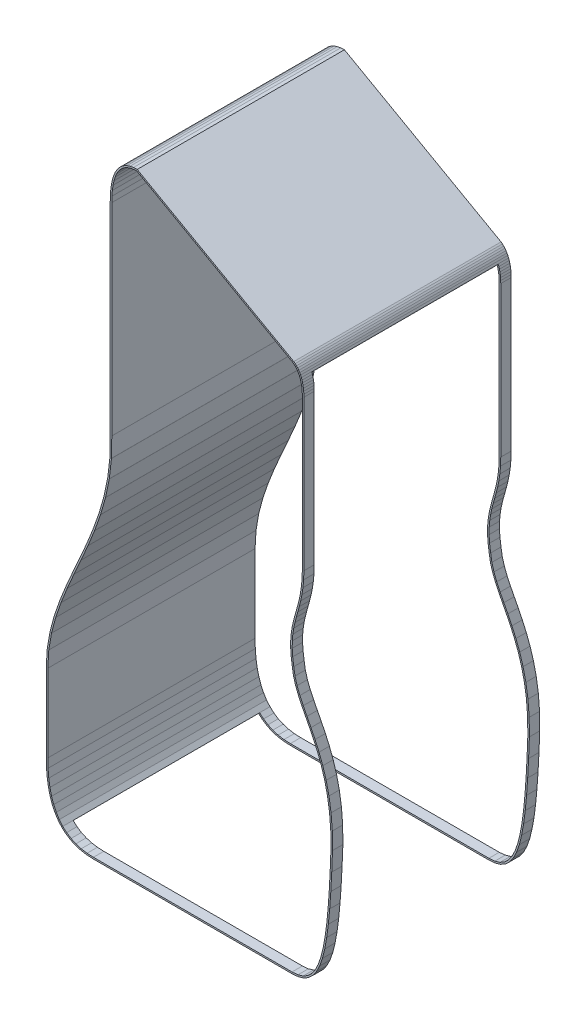
SolidWorks part; units mm, degrees
ref_plane "前视基准面" through (0, 0, 0) normal (0, 0, 1) x (1, 0, 0)
ref_plane "上视基准面" through (0, 0, 0) normal (0, 1, 0) x (1, 0, 0)
ref_plane "右视基准面" through (0, 0, 0) normal (1, 0, 0) x (0, 0, -1)
other "Configuration Table"
sketch "草图1" plane through (0, 0, 0) normal (0, 0, 1) x (1, 0, 0)
  line L0 (103, 235) -> (-24.8333, 235)
  line L1 (-24.8333, 235) -> (-152.6667, 235)
  line L2 (-152.6667, 235) -> (-280.5, 235)
  line L3 (-280.5, 235) -> (-293.0357, 235.6378)
  line L4 (-293.0357, 235.6378) -> (-304.6429, 237.551)
  line L5 (-304.6429, 237.551) -> (-315.3214, 240.7398)
  line L6 (-315.3214, 240.7398) -> (-325.0714, 245.2041)
  line L7 (-325.0714, 245.2041) -> (-333.8929, 250.9439)
  line L8 (-333.8929, 250.9439) -> (-341.7857, 257.9592)
  line L9 (-341.7857, 257.9592) -> (-348.75, 266.25)
  line L10 (-348.75, 266.25) -> (-354.7857, 275.8163)
  line L11 (-354.7857, 275.8163) -> (-359.8929, 286.6582)
  line L12 (-359.8929, 286.6582) -> (-364.0714, 298.7755)
  line L13 (-364.0714, 298.7755) -> (-367.3214, 312.1684)
  line L14 (-367.3214, 312.1684) -> (-369.6429, 326.8367)
  line L15 (-369.6429, 326.8367) -> (-371.0357, 342.7806)
  line L16 (-371.0357, 342.7806) -> (-371.5, 360)
  line L17 (-371.5, 360) -> (-371.5, 410)
  line L18 (-371.5, 410) -> (-371.5, 460)
  line L19 (-371.5, 460) -> (-371.5, 510)
  line L20 (-371.5, 510) -> (-369.6073, 541.7165)
  line L21 (-369.6073, 541.7165) -> (-364.3178, 572.7114)
  line L22 (-364.3178, 572.7114) -> (-356.2141, 603.1815)
  line L23 (-356.2141, 603.1815) -> (-345.879, 633.3236)
  line L24 (-345.879, 633.3236) -> (-333.8952, 663.3345)
  line L25 (-333.8952, 663.3345) -> (-320.8455, 693.4111)
  line L26 (-320.8455, 693.4111) -> (-307.3125, 723.75)
  line L27 (-307.3125, 723.75) -> (-293.879, 754.5481)
  line L28 (-293.879, 754.5481) -> (-281.1277, 786.0022)
  line L29 (-281.1277, 786.0022) -> (-269.6414, 818.309)
  line L30 (-269.6414, 818.309) -> (-260.0027, 851.6655)
  line L31 (-260.0027, 851.6655) -> (-252.7945, 886.2682)
  line L32 (-252.7945, 886.2682) -> (-248.5993, 922.3141)
  line L33 (-248.5993, 922.3141) -> (-248, 960)
  line L34 (-248, 960) -> (-248, 1090)
  line L35 (-248, 1090) -> (-248, 1220)
  line L36 (-248, 1220) -> (-248, 1350)
  line L37 (-248, 1350) -> (-247.7347, 1361.0204)
  line L38 (-247.7347, 1361.0204) -> (-246.9388, 1371.2245)
  line L39 (-246.9388, 1371.2245) -> (-245.6122, 1380.6122)
  line L40 (-245.6122, 1380.6122) -> (-243.7551, 1389.1837)
  line L41 (-243.7551, 1389.1837) -> (-241.3673, 1396.9388)
  line L42 (-241.3673, 1396.9388) -> (-238.449, 1403.8776)
  line L43 (-238.449, 1403.8776) -> (-235, 1410)
  line L44 (-235, 1410) -> (-231.0204, 1415.3061)
  line L45 (-231.0204, 1415.3061) -> (-226.5102, 1419.7959)
  line L46 (-226.5102, 1419.7959) -> (-221.4694, 1423.4694)
  line L47 (-221.4694, 1423.4694) -> (-215.898, 1426.3265)
  line L48 (-215.898, 1426.3265) -> (-209.7959, 1428.3673)
  line L49 (-209.7959, 1428.3673) -> (-203.1633, 1429.5918)
  line L50 (-203.1633, 1429.5918) -> (-196, 1430)
  line L51 (-196, 1430) -> (-95.25, 1373.3333)
  line L52 (-95.25, 1373.3333) -> (5.5, 1316.6667)
  line L53 (5.5, 1316.6667) -> (106.25, 1260)
  line L54 (106.25, 1260) -> (108.9362, 1257.8878)
  line L55 (108.9362, 1257.8878) -> (111.4235, 1255.551)
  line L56 (111.4235, 1255.551) -> (113.7117, 1252.9898)
  line L57 (113.7117, 1252.9898) -> (115.801, 1250.2041)
  line L58 (115.801, 1250.2041) -> (117.6913, 1247.1939)
  line L59 (117.6913, 1247.1939) -> (119.3827, 1243.9592)
  line L60 (119.3827, 1243.9592) -> (120.875, 1240.5)
  line L61 (120.875, 1240.5) -> (122.1684, 1236.8163)
  line L62 (122.1684, 1236.8163) -> (123.2628, 1232.9082)
  line L63 (123.2628, 1232.9082) -> (124.1582, 1228.7755)
  line L64 (124.1582, 1228.7755) -> (124.8546, 1224.4184)
  line L65 (124.8546, 1224.4184) -> (125.352, 1219.8367)
  line L66 (125.352, 1219.8367) -> (125.6505, 1215.0306)
  line L67 (125.6505, 1215.0306) -> (125.75, 1210)
  line L68 (125.75, 1210) -> (125.75, 1113.3333)
  line L69 (125.75, 1113.3333) -> (125.75, 1016.6667)
  line L70 (125.75, 1016.6667) -> (125.75, 920)
  line L71 (125.75, 920) -> (125.281, 904.7303)
  line L72 (125.281, 904.7303) -> (123.9876, 890.9038)
  line L73 (123.9876, 890.9038) -> (122.0405, 878.2799)
  line L74 (122.0405, 878.2799) -> (119.6101, 866.6181)
  line L75 (119.6101, 866.6181) -> (116.867, 855.6778)
  line L76 (116.867, 855.6778) -> (113.9818, 845.2187)
  line L77 (113.9818, 845.2187) -> (111.125, 835)
  line L78 (111.125, 835) -> (108.4672, 824.7813)
  line L79 (108.4672, 824.7813) -> (106.1789, 814.3222)
  line L80 (106.1789, 814.3222) -> (104.4308, 803.3819)
  line L81 (104.4308, 803.3819) -> (103.3932, 791.7201)
  line L82 (103.3932, 791.7201) -> (103.2369, 779.0962)
  line L83 (103.2369, 779.0962) -> (104.1323, 765.2697)
  line L84 (104.1323, 765.2697) -> (106.25, 750)
  line L85 (106.25, 750) -> (108.5868, 735.4045)
  line L86 (108.5868, 735.4045) -> (112.6079, 721.3994)
  line L87 (112.6079, 721.3994) -> (118.0076, 707.6567)
  line L88 (118.0076, 707.6567) -> (124.4803, 693.8484)
  line L89 (124.4803, 693.8484) -> (131.7206, 679.6465)
  line L90 (131.7206, 679.6465) -> (139.4227, 664.723)
  line L91 (139.4227, 664.723) -> (147.2812, 648.75)
  line L92 (147.2812, 648.75) -> (154.9905, 631.3994)
  line L93 (154.9905, 631.3994) -> (162.245, 612.3433)
  line L94 (162.245, 612.3433) -> (168.7391, 591.2536)
  line L95 (168.7391, 591.2536) -> (174.1672, 567.8025)
  line L96 (174.1672, 567.8025) -> (178.2238, 541.6618)
  line L97 (178.2238, 541.6618) -> (180.6032, 512.5036)
  line L98 (180.6032, 512.5036) -> (181, 480)
  line L99 (181, 480) -> (179.4934, 443.1706)
  line L100 (179.4934, 443.1706) -> (177.7026, 409.7522)
  line L101 (177.7026, 409.7522) -> (175.5423, 379.6356)
  line L102 (175.5423, 379.6356) -> (172.9271, 352.7114)
  line L103 (172.9271, 352.7114) -> (169.7719, 328.8703)
  line L104 (169.7719, 328.8703) -> (165.9913, 308.0029)
  line L105 (165.9913, 308.0029) -> (161.5, 290)
  line L106 (161.5, 290) -> (156.2128, 274.7522)
  line L107 (156.2128, 274.7522) -> (150.0445, 262.1501)
  line L108 (150.0445, 262.1501) -> (142.9096, 252.0845)
  line L109 (142.9096, 252.0845) -> (134.723, 244.4461)
  line L110 (134.723, 244.4461) -> (125.3994, 239.1254)
  line L111 (125.3994, 239.1254) -> (114.8535, 236.0131)
  line L112 (114.8535, 236.0131) -> (103, 235)
  line L113 (102.872, 238) -> (-280.4237, 238)
  line L114 (-280.4237, 238) -> (-292.7145, 238.6253)
  line L115 (-292.7145, 238.6253) -> (-303.967, 240.4801)
  line L116 (-303.967, 240.4801) -> (-314.2626, 243.5545)
  line L117 (-314.2626, 243.5545) -> (-323.621, 247.8395)
  line L118 (-323.621, 247.8395) -> (-332.0681, 253.3357)
  line L119 (-332.0681, 253.3357) -> (-339.6293, 260.0562)
  line L120 (-339.6293, 260.0562) -> (-346.3217, 268.0234)
  line L121 (-346.3217, 268.0234) -> (-352.1502, 277.2614)
  line L122 (-352.1502, 277.2614) -> (-357.1097, 287.7897)
  line L123 (-357.1097, 287.7897) -> (-361.1893, 299.6201)
  line L124 (-361.1893, 299.6201) -> (-364.3773, 312.7575)
  line L125 (-364.3773, 312.7575) -> (-366.6634, 327.2022)
  line L126 (-366.6634, 327.2022) -> (-368.0392, 342.9517)
  line L127 (-368.0392, 342.9517) -> (-368.5, 360.0404)
  line L128 (-368.5, 360.0404) -> (-368.5, 509.9106)
  line L129 (-368.5, 509.9106) -> (-366.6224, 541.3738)
  line L130 (-366.6224, 541.3738) -> (-361.3835, 572.0722)
  line L131 (-361.3835, 572.0722) -> (-353.342, 602.3084)
  line L132 (-353.342, 602.3084) -> (-343.0653, 632.2802)
  line L133 (-343.0653, 632.2802) -> (-331.1255, 662.181)
  line L134 (-331.1255, 662.181) -> (-318.0995, 692.2029)
  line L135 (-318.0995, 692.2029) -> (-304.5727, 722.5279)
  line L136 (-304.5727, 722.5279) -> (-304.5627, 722.5506)
  line L137 (-304.5627, 722.5506) -> (-291.1292, 753.3487)
  line L138 (-291.1292, 753.3487) -> (-291.0988, 753.421)
  line L139 (-291.0988, 753.421) -> (-278.3475, 784.8751)
  line L140 (-278.3475, 784.8751) -> (-278.3011, 784.9972)
  line L141 (-278.3011, 784.9972) -> (-266.8147, 817.3041)
  line L142 (-266.8147, 817.3041) -> (-266.7593, 817.4762)
  line L143 (-266.7593, 817.4762) -> (-257.1206, 850.8326)
  line L144 (-257.1206, 850.8326) -> (-257.0658, 851.0536)
  line L145 (-257.0658, 851.0536) -> (-249.8575, 885.6564)
  line L146 (-249.8575, 885.6564) -> (-249.8146, 885.9214)
  line L147 (-249.8146, 885.9214) -> (-245.6194, 921.9673)
  line L148 (-245.6194, 921.9673) -> (-245.5997, 922.2664)
  line L149 (-245.5997, 922.2664) -> (-245.0004, 959.9523)
  line L150 (-245.0004, 959.9523) -> (-245, 960)
  line L151 (-245, 960) -> (-245, 1349.9639)
  line L152 (-245, 1349.9639) -> (-244.7375, 1360.8676)
  line L153 (-244.7375, 1360.8676) -> (-243.9552, 1370.8977)
  line L154 (-243.9552, 1370.8977) -> (-242.6571, 1380.084)
  line L155 (-242.6571, 1380.084) -> (-240.8502, 1388.4233)
  line L156 (-240.8502, 1388.4233) -> (-238.5441, 1395.9133)
  line L157 (-238.5441, 1395.9133) -> (-235.7505, 1402.5554)
  line L158 (-235.7505, 1402.5554) -> (-232.4824, 1408.3568)
  line L159 (-232.4824, 1408.3568) -> (-228.7504, 1413.3328)
  line L160 (-228.7504, 1413.3328) -> (-224.5571, 1417.5072)
  line L161 (-224.5571, 1417.5072) -> (-219.8919, 1420.9069)
  line L162 (-219.8919, 1420.9069) -> (-214.7311, 1423.5535)
  line L163 (-214.7311, 1423.5535) -> (-209.0441, 1425.4554)
  line L164 (-209.0441, 1425.4554) -> (-202.8042, 1426.6074)
  line L165 (-202.8042, 1426.6074) -> (-196.7057, 1426.9549)
  line L166 (-196.7057, 1426.9549) -> (-96.7207, 1370.7185)
  line L167 (-96.7207, 1370.7185) -> (104.5776, 1257.4987)
  line L168 (104.5776, 1257.4987) -> (106.9782, 1255.611)
  line L169 (106.9782, 1255.611) -> (109.2737, 1253.4544)
  line L170 (109.2737, 1253.4544) -> (111.3889, 1251.0869)
  line L171 (111.3889, 1251.0869) -> (113.3265, 1248.5035)
  line L172 (113.3265, 1248.5035) -> (115.0877, 1245.6988)
  line L173 (115.0877, 1245.6988) -> (116.6723, 1242.6682)
  line L174 (116.6723, 1242.6682) -> (118.079, 1239.4076)
  line L175 (118.079, 1239.4076) -> (119.3056, 1235.914)
  line L176 (119.3056, 1235.914) -> (120.3497, 1232.1854)
  line L177 (120.3497, 1232.1854) -> (121.2088, 1228.2207)
  line L178 (121.2088, 1228.2207) -> (121.8803, 1224.0195)
  line L179 (121.8803, 1224.0195) -> (122.3621, 1219.5817)
  line L180 (122.3621, 1219.5817) -> (122.6523, 1214.9079)
  line L181 (122.6523, 1214.9079) -> (122.75, 1209.9703)
  line L182 (122.75, 1209.9703) -> (122.75, 920.0461)
  line L183 (122.75, 920.0461) -> (122.2853, 904.9163)
  line L184 (122.2853, 904.9163) -> (121.009, 891.2725)
  line L185 (121.009, 891.2725) -> (119.0875, 878.8149)
  line L186 (119.0875, 878.8149) -> (116.6855, 867.2892)
  line L187 (116.6855, 867.2892) -> (113.9656, 856.4416)
  line L188 (113.9656, 856.4416) -> (111.0912, 846.0214)
  line L189 (111.0912, 846.0214) -> (108.2358, 835.8077)
  line L190 (108.2358, 835.8077) -> (108.2216, 835.7552)
  line L191 (108.2216, 835.7552) -> (105.5638, 825.5365)
  line L192 (105.5638, 825.5365) -> (105.5365, 825.4225)
  line L193 (105.5365, 825.4225) -> (103.2483, 814.9633)
  line L194 (103.2483, 814.9633) -> (103.2165, 814.7955)
  line L195 (103.2165, 814.7955) -> (101.4683, 803.8553)
  line L196 (101.4683, 803.8553) -> (101.4426, 803.6478)
  line L197 (101.4426, 803.6478) -> (100.405, 791.986)
  line L198 (100.405, 791.986) -> (100.3935, 791.7573)
  line L199 (100.3935, 791.7573) -> (100.2371, 779.1334)
  line L200 (100.2371, 779.1334) -> (100.2432, 778.9023)
  line L201 (100.2432, 778.9023) -> (101.1386, 765.0758)
  line L202 (101.1386, 765.0758) -> (101.1607, 764.8576)
  line L203 (101.1607, 764.8576) -> (103.2784, 749.5879)
  line L204 (103.2784, 749.5879) -> (103.2877, 749.5257)
  line L205 (103.2877, 749.5257) -> (105.6246, 734.9302)
  line L206 (105.6246, 734.9302) -> (105.7033, 734.5766)
  line L207 (105.7033, 734.5766) -> (109.7244, 720.5715)
  line L208 (109.7244, 720.5715) -> (109.8157, 720.3023)
  line L209 (109.8157, 720.3023) -> (115.2154, 706.5596)
  line L210 (115.2154, 706.5596) -> (115.2912, 706.3834)
  line L211 (115.2912, 706.3834) -> (121.764, 692.5751)
  line L212 (121.764, 692.5751) -> (121.8076, 692.4858)
  line L213 (121.8076, 692.4858) -> (129.0479, 678.2839)
  line L214 (129.0479, 678.2839) -> (129.0547, 678.2706)
  line L215 (129.0547, 678.2706) -> (136.7436, 663.3728)
  line L216 (136.7436, 663.3728) -> (144.5635, 647.4783)
  line L217 (144.5635, 647.4783) -> (152.2158, 630.2558)
  line L218 (152.2158, 630.2558) -> (159.4066, 611.3672)
  line L219 (159.4066, 611.3672) -> (165.8405, 590.473)
  line L220 (165.8405, 590.473) -> (171.2196, 567.2334)
  line L221 (171.2196, 567.2334) -> (175.2426, 541.3093)
  line L222 (175.2426, 541.3093) -> (177.6047, 512.3632)
  line L223 (177.6047, 512.3632) -> (177.9993, 480.043)
  line L224 (177.9993, 480.043) -> (176.4967, 443.3121)
  line L225 (176.4967, 443.3121) -> (174.7084, 409.9398)
  line L226 (174.7084, 409.9398) -> (172.5527, 379.8879)
  line L227 (172.5527, 379.8879) -> (169.9462, 353.0533)
  line L228 (169.9462, 353.0533) -> (166.8072, 329.3347)
  line L229 (166.8072, 329.3347) -> (163.0568, 308.6341)
  line L230 (163.0568, 308.6341) -> (158.6217, 290.8562)
  line L231 (158.6217, 290.8562) -> (153.4381, 275.9073)
  line L232 (153.4381, 275.9073) -> (147.4566, 263.687)
  line L233 (147.4566, 263.687) -> (140.6392, 254.0692)
  line L234 (140.6392, 254.0692) -> (132.9322, 246.8782)
  line L235 (132.9322, 246.8782) -> (124.2156, 241.9039)
  line L236 (124.2156, 241.9039) -> (114.2955, 238.9764)
  line L237 (114.2955, 238.9764) -> (102.872, 238)
  point P0 (0, 0)
  dimension "D1" = 0.4643
  dimension "D2" = 1.8571
  dimension "D3" = 1.8927
  dimension "D4" = 3
  dimension "D5" = 3.4608
  dimension "D6" = 4.1786
  dimension "D7" = 4.8366
  dimension "D8" = 4.8776
  dimension "D9" = 7.1227
  dimension "D10" = 7.1822
  dimension "D11" = 7.4286
  dimension "D12" = 10.1165
  dimension "D13" = 10.3107
  dimension "D14" = 11.6071
  dimension "D15" = 14.3903
  dimension "D16" = 15.2859
  dimension "D17" = 16.7143
  dimension "D18" = 18.158
  dimension "D19" = 19.3498
  dimension "D20" = 22.75
  dimension "D21" = 25.1783
  dimension "D22" = 25.621
  dimension "D23" = 28.4347
  dimension "D24" = 29.7143
  dimension "D25" = 31.8707
  dimension "D26" = 37.6048
  dimension "D27" = 37.6071
  dimension "D28" = 39.4319
  dimension "D29" = 40.3745
  dimension "D30" = 46.4286
  dimension "D31" = 47.879
  dimension "D32" = 50.6545
  dimension "D33" = 53.4005
  dimension "D34" = 56.1786
  dimension "D35" = 57.2374
  dimension "D36" = 64.1875
  dimension "D37" = 66.8571
  dimension "D38" = 66.9273
  dimension "D39" = 66.9373
  dimension "D40" = 67.533
  dimension "D41" = 77.621
  dimension "D42" = 78.4643
  dimension "D43" = 78.7855
  dimension "D44" = 80.3708
  dimension "D45" = 80.4012
  dimension "D46" = 90.3723
  dimension "D47" = 91
  dimension "D48" = 91.0763
  dimension "D49" = 93.1525
  dimension "D50" = 93.1989
  dimension "D51" = 101.8586
  dimension "D52" = 104.6853
  dimension "D53" = 104.7407
  dimension "D54" = 111.4973
  dimension "D55" = 114.3794
  dimension "D56" = 114.4342
  dimension "D57" = 118.7055
  dimension "D58" = 121.6425
  dimension "D59" = 121.6854
  dimension "D60" = 122.9007
  dimension "D61" = 123.5
  dimension "D62" = 123.7653
  dimension "D63" = 124.5612
  dimension "D64" = 125.8806
  dimension "D65" = 125.8878
  dimension "D66" = 125.9003
  dimension "D67" = 126.4996
  dimension "D68" = 126.5
  dimension "D69" = 126.7625
  dimension "D70" = 127.5448
  dimension "D71" = 127.7449
  dimension "D72" = 128.8429
  dimension "D73" = 130.1327
  dimension "D74" = 130.6498
  dimension "D75" = 132.9559
  dimension "D76" = 133.051
  dimension "D77" = 135.7495
  dimension "D78" = 136.5
  dimension "D79" = 139.0176
  dimension "D80" = 140.4796
  dimension "D81" = 142.7496
  dimension "D82" = 144.9898
  dimension "D83" = 146.9429
  dimension "D84" = 150.0306
  dimension "D85" = 151.6081
  dimension "D86" = 155.602
  dimension "D87" = 156.7689
  dimension "D88" = 161.7041
  dimension "D89" = 162.4559
  dimension "D90" = 168.3367
  dimension "D91" = 168.6958
  dimension "D92" = 174.7943
  dimension "D93" = 175.5
  dimension "D94" = 218.8333
  dimension "D95" = 274.7793
  dimension "D96" = 276.25
  dimension "D97" = 346.6667
  dimension "D98" = 371.5
  dimension "D99" = 377
  dimension "D100" = 471.7371
  dimension "D101" = 471.7432
  dimension "D102" = 471.8935
  dimension "D103" = 471.905
  dimension "D104" = 472.6386
  dimension "D105" = 472.6607
  dimension "D106" = 472.9426
  dimension "D107" = 472.9683
  dimension "D108" = 474.372
  dimension "D109" = 474.5
  dimension "D110" = 474.7165
  dimension "D111" = 474.7369
  dimension "D112" = 474.7483
  dimension "D113" = 474.7784
  dimension "D114" = 474.7877
  dimension "D115" = 474.8932
  dimension "D116" = 475.6323
  dimension "D117" = 475.9308
  dimension "D118" = 476.0776
  dimension "D119" = 477.0365
  dimension "D120" = 477.0638
  dimension "D121" = 477.1246
  dimension "D122" = 477.2033
  dimension "D123" = 477.6789
  dimension "D124" = 477.75
  dimension "D125" = 478.4782
  dimension "D126" = 479.7216
  dimension "D127" = 479.7358
  dimension "D128" = 479.9672
  dimension "D129" = 480.0868
  dimension "D130" = 480.4362
  dimension "D131" = 480.7737
  dimension "D132" = 481.2244
  dimension "D133" = 481.3157
  dimension "D134" = 482.5912
  dimension "D135" = 482.625
  dimension "D136" = 482.8889
  dimension "D137" = 482.9235
  dimension "D138" = 484.1079
  dimension "D139" = 484.8265
  dimension "D140" = 485.2117
  dimension "D141" = 485.4656
  dimension "D142" = 485.4818
  dimension "D143" = 485.7955
  dimension "D144" = 486.3535
  dimension "D145" = 486.5877
  dimension "D146" = 486.7154
  dimension "D147" = 486.7912
  dimension "D148" = 487.301
  dimension "D149" = 488.1723
  dimension "D150" = 488.1855
  dimension "D151" = 488.367
  dimension "D152" = 489.1913
  dimension "D153" = 489.5076
  dimension "D154" = 489.579
  dimension "D155" = 490.5875
  dimension "D156" = 490.8056
  dimension "D157" = 490.8827
  dimension "D158" = 491.1101
  dimension "D159" = 491.8497
  dimension "D160" = 492.375
  dimension "D161" = 492.509
  dimension "D162" = 492.7088
  dimension "D163" = 493.264
  dimension "D164" = 493.3076
  dimension "D165" = 493.3803
  dimension "D166" = 493.5405
  dimension "D167" = 493.6684
  dimension "D168" = 493.7853
  dimension "D169" = 493.8621
  dimension "D170" = 494.1523
  dimension "D171" = 494.25
  dimension "D172" = 494.7628
  dimension "D173" = 495.4876
  dimension "D174" = 495.6582
  dimension "D175" = 495.7156
  dimension "D176" = 495.9803
  dimension "D177" = 496.3546
  dimension "D178" = 496.781
  dimension "D179" = 496.852
  dimension "D180" = 496.8994
  dimension "D181" = 497.1505
  dimension "D182" = 497.25
  dimension "D183" = 500.5479
  dimension "D184" = 500.5547
  dimension "D185" = 503.2206
  dimension "D186" = 504.4322
  dimension "D187" = 506.223
  dimension "D188" = 508.2436
  dimension "D189" = 510.9227
  dimension "D190" = 512.1392
  dimension "D191" = 514.4096
  dimension "D192" = 516.0635
  dimension "D193" = 518.7812
  dimension "D194" = 518.9566
  dimension "D195" = 521.5445
  dimension "D196" = 523.7158
  dimension "D197" = 524.9381
  dimension "D198" = 526.4905
  dimension "D199" = 527.7128
  dimension "D200" = 530.1217
  dimension "D201" = 530.9066
  dimension "D202" = 533
  dimension "D203" = 533.745
  dimension "D204" = 534.5568
  dimension "D205" = 537.3405
  dimension "D206" = 537.4913
  dimension "D207" = 538.3072
  dimension "D208" = 540.2391
  dimension "D209" = 541.2719
  dimension "D210" = 541.4462
  dimension "D211" = 542.7196
  dimension "D212" = 544.0527
  dimension "D213" = 544.4271
  dimension "D214" = 545.6672
  dimension "D215" = 546.2084
  dimension "D216" = 546.7426
  dimension "D217" = 547.0423
  dimension "D218" = 547.9967
  dimension "D219" = 549.1047
  dimension "D220" = 549.2026
  dimension "D221" = 549.4993
  dimension "D222" = 549.7238
  dimension "D223" = 550.9934
  dimension "D224" = 552.1032
  dimension "D225" = 552.5
  dimension "D226" = 0.6378
  dimension "D227" = 1.0131
  dimension "D228" = 2.551
  dimension "D229" = 3
  dimension "D230" = 3.6253
  dimension "D231" = 3.9764
  dimension "D232" = 4.1254
  dimension "D233" = 5.4801
  dimension "D234" = 5.7398
  dimension "D235" = 6.9039
  dimension "D236" = 8.5545
  dimension "D237" = 9.4461
  dimension "D238" = 10.2041
  dimension "D239" = 11.8782
  dimension "D240" = 12.8395
  dimension "D241" = 15.9439
  dimension "D242" = 17.0845
  dimension "D243" = 18.3357
  dimension "D244" = 19.0692
  dimension "D245" = 22.9592
  dimension "D246" = 25.0562
  dimension "D247" = 27.1501
  dimension "D248" = 28.687
  dimension "D249" = 31.25
  dimension "D250" = 33.0234
  dimension "D251" = 39.7522
  dimension "D252" = 40.8163
  dimension "D253" = 40.9073
  dimension "D254" = 42.2614
  dimension "D255" = 51.6582
  dimension "D256" = 52.7897
  dimension "D257" = 55
  dimension "D258" = 55.8562
  dimension "D259" = 63.7755
  dimension "D260" = 64.6201
  dimension "D261" = 73.0029
  dimension "D262" = 73.6341
  dimension "D263" = 77.1684
  dimension "D264" = 77.7575
  dimension "D265" = 91.8367
  dimension "D266" = 92.2022
  dimension "D267" = 93.8703
  dimension "D268" = 94.3347
  dimension "D269" = 107.7806
  dimension "D270" = 107.9517
  dimension "D271" = 117.7114
  dimension "D272" = 118.0533
  dimension "D273" = 125
  dimension "D274" = 125.0404
  dimension "D275" = 144.6356
  dimension "D276" = 144.8879
  dimension "D277" = 174.7522
  dimension "D278" = 174.9398
  dimension "D279" = 175
  dimension "D280" = 208.1706
  dimension "D281" = 208.3121
  dimension "D282" = 225
  dimension "D283" = 245
  dimension "D284" = 245.043
  dimension "D285" = 274.9106
  dimension "D286" = 275
  dimension "D287" = 277.3632
  dimension "D288" = 277.5036
  dimension "D289" = 306.3093
  dimension "D290" = 306.3738
  dimension "D291" = 306.6618
  dimension "D292" = 306.7165
  dimension "D293" = 332.2334
  dimension "D294" = 332.8025
  dimension "D295" = 337.0722
  dimension "D296" = 337.7114
  dimension "D297" = 355.473
  dimension "D298" = 356.2536
  dimension "D299" = 367.3084
  dimension "D300" = 368.1815
  dimension "D301" = 376.3672
  dimension "D302" = 377.3433
  dimension "D303" = 395.2558
  dimension "D304" = 396.3994
  dimension "D305" = 397.2802
  dimension "D306" = 398.3236
  dimension "D307" = 412.4783
  dimension "D308" = 413.75
  dimension "D309" = 427.181
  dimension "D310" = 428.3345
  dimension "D311" = 428.3728
  dimension "D312" = 429.723
  dimension "D313" = 443.2706
  dimension "D314" = 443.2839
  dimension "D315" = 444.6465
  dimension "D316" = 457.2029
  dimension "D317" = 457.4858
  dimension "D318" = 457.5751
  dimension "D319" = 458.4111
  dimension "D320" = 458.8484
  dimension "D321" = 471.3834
  dimension "D322" = 471.5596
  dimension "D323" = 472.6567
  dimension "D324" = 485.3023
  dimension "D325" = 485.5715
  dimension "D326" = 486.3994
  dimension "D327" = 487.5279
  dimension "D328" = 487.5506
  dimension "D329" = 488.75
  dimension "D330" = 499.5766
  dimension "D331" = 499.9302
  dimension "D332" = 500.4045
  dimension "D333" = 514.5257
  dimension "D334" = 514.5879
  dimension "D335" = 515
  dimension "D336" = 518.3487
  dimension "D337" = 518.421
  dimension "D338" = 519.5481
  dimension "D339" = 529.8576
  dimension "D340" = 530.0758
  dimension "D341" = 530.2697
  dimension "D342" = 543.9023
  dimension "D343" = 544.0962
  dimension "D344" = 544.1334
  dimension "D345" = 549.8751
  dimension "D346" = 549.9972
  dimension "D347" = 551.0022
  dimension "D348" = 556.7201
  dimension "D349" = 556.7573
  dimension "D350" = 556.986
  dimension "D351" = 568.3819
  dimension "D352" = 568.6478
  dimension "D353" = 568.8553
  dimension "D354" = 579.3222
  dimension "D355" = 579.7955
  dimension "D356" = 579.9633
  dimension "D357" = 582.3041
  dimension "D358" = 582.4762
  dimension "D359" = 583.309
  dimension "D360" = 589.7813
  dimension "D361" = 590.4225
  dimension "D362" = 590.5365
  dimension "D363" = 600
  dimension "D364" = 600.7552
  dimension "D365" = 600.8077
  dimension "D366" = 610.2187
  dimension "D367" = 611.0214
  dimension "D368" = 615.8326
  dimension "D369" = 616.0536
  dimension "D370" = 616.6655
  dimension "D371" = 620.6778
  dimension "D372" = 621.4416
  dimension "D373" = 631.6181
  dimension "D374" = 632.2892
  dimension "D375" = 643.2799
  dimension "D376" = 643.8149
  dimension "D377" = 650.6564
  dimension "D378" = 650.9214
  dimension "D379" = 651.2682
  dimension "D380" = 655.9038
  dimension "D381" = 656.2725
  dimension "D382" = 669.7303
  dimension "D383" = 669.9163
  dimension "D384" = 685
  dimension "D385" = 685.0461
  dimension "D386" = 686.9673
  dimension "D387" = 687.2664
  dimension "D388" = 687.3141
  dimension "D389" = 724.9523
  dimension "D390" = 725
  dimension "D391" = 781.6667
  dimension "D392" = 855
  dimension "D393" = 878.3333
  dimension "D394" = 974.9703
  dimension "D395" = 975
  dimension "D396" = 979.9079
  dimension "D397" = 980.0306
  dimension "D398" = 984.5817
  dimension "D399" = 984.8367
  dimension "D400" = 985
  dimension "D401" = 989.0195
  dimension "D402" = 989.4184
  dimension "D403" = 993.2207
  dimension "D404" = 993.7755
  dimension "D405" = 997.1854
  dimension "D406" = 997.9082
  dimension "D407" = 1000.914
  dimension "D408" = 1001.8163
  dimension "D409" = 1004.4076
  dimension "D410" = 1005.5
  dimension "D411" = 1007.6682
  dimension "D412" = 1008.9592
  dimension "D413" = 1010.6988
  dimension "D414" = 1012.1939
  dimension "D415" = 1013.5035
  dimension "D416" = 1015.2041
  dimension "D417" = 1016.0869
  dimension "D418" = 1017.9898
  dimension "D419" = 1018.4544
  dimension "D420" = 1020.551
  dimension "D421" = 1020.611
  dimension "D422" = 1022.4987
  dimension "D423" = 1022.8878
  dimension "D424" = 1025
  dimension "D425" = 1081.6667
  dimension "D426" = 1114.9639
  dimension "D427" = 1115
  dimension "D428" = 1125.8676
  dimension "D429" = 1126.0204
  dimension "D430" = 1135.7185
  dimension "D431" = 1135.8977
  dimension "D432" = 1136.2245
  dimension "D433" = 235
  dimension "D434" = 1145.084
  dimension "D435" = 1145.6122
  dimension "D436" = 1153.4233
  dimension "D437" = 1154.1837
  dimension "D438" = 1160.9133
  dimension "D439" = 1161.9388
  dimension "D440" = 1167.5554
  dimension "D441" = 1168.8776
  dimension "D442" = 1173.3568
  dimension "D443" = 1175
  dimension "D444" = 1178.3328
  dimension "D445" = 1180.3061
  dimension "D446" = 1182.5072
  dimension "D447" = 1184.7959
  dimension "D448" = 1185.9069
  dimension "D449" = 1188.4694
  dimension "D450" = 1188.5535
  dimension "D451" = 1190.4554
  dimension "D452" = 1191.3265
  dimension "D453" = 1191.6074
  dimension "D455" = 1193.3673
  dimension "D456" = 1194.5918
extrude "凸台-拉伸1" add sketch "草图1" against normal mid plane 400
sketch "草图2" plane through (0, 0, 0) normal (0, 0, 1) x (1, 0, 0)
  line L0 (60, 220) -> (240, 220)
  line L1 (240, 220) -> (240, 1240)
  line L2 (240, 1240) -> (60, 1240)
  line L3 (60, 1240) -> (60, 220)
  point P0 (0, 0)
  dimension "D1" = 180
  dimension "D2" = 240
  dimension "D3" = 1020
  dimension "D4" = 1240
extrude "切除-拉伸1" cut sketch "草图2" against normal mid plane 360
sketch "草图3" plane through (0, 0, 0) normal (0, 0, 1) x (1, 0, 0)
  line L0 (-600, 220) -> (100, 220)
  line L1 (100, 220) -> (100, 260)
  line L2 (100, 260) -> (-600, 260)
  line L3 (-600, 260) -> (-600, 220)
  point P0 (0, 0)
  dimension "D1" = 100
  dimension "D2" = 700
  dimension "D3" = 40
  dimension "D4" = 260
extrude "切除-拉伸2" cut sketch "草图3" against normal mid plane 360
